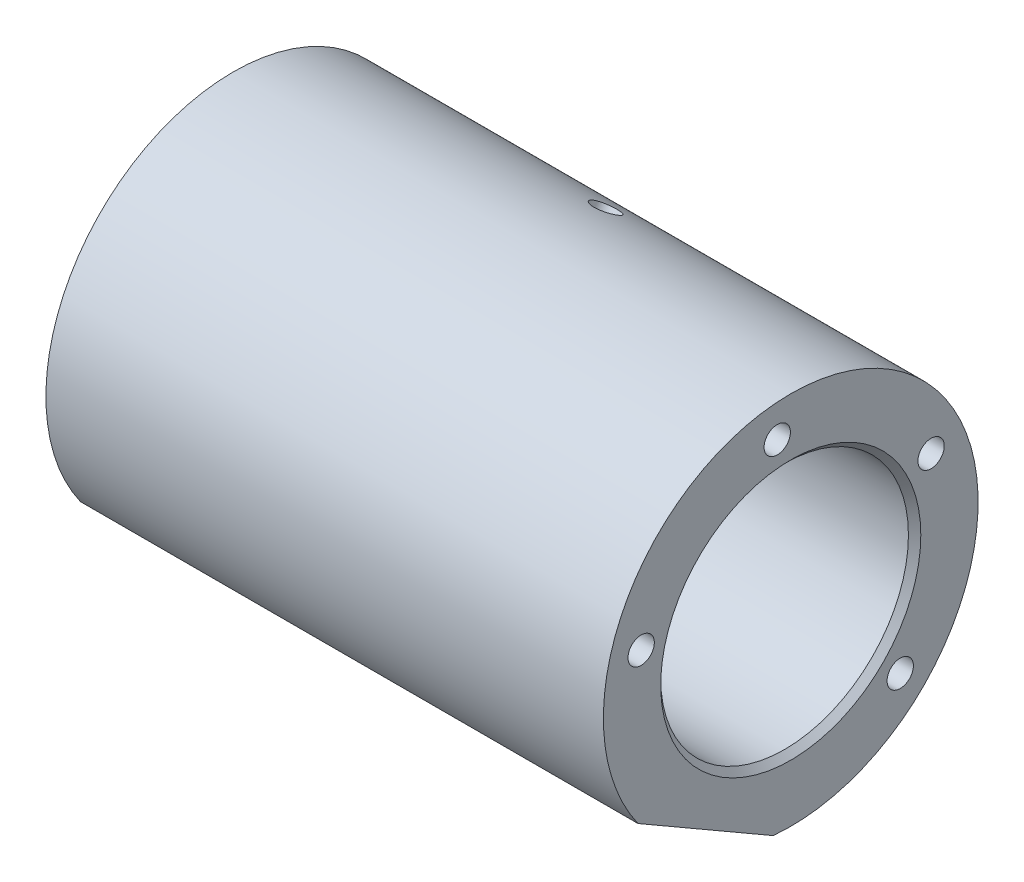
SolidWorks part; units mm, degrees
material "Q345B"
ref_plane "Front Plane" through (0, 0, 0) normal (0, 0, 1) x (1, 0, 0)
ref_plane "Top Plane" through (0, 0, 0) normal (0, 1, 0) x (1, 0, 0)
ref_plane "Right Plane" through (0, 0, 0) normal (1, 0, 0) x (0, 0, -1)
sketch "Sketch1" plane through (0, 0, 0) normal (1, 0, 0) x (0, 0, -1)
  circle A0 centre (0, 0) radius 60.5
  circle A1 centre (0, 0) radius 40
  dimension "D1" = 121
  dimension "D2" = 80
extrude "Boss-Extrude1" add sketch "Sketch1" along normal mid plane 180
sketch "Sketch5" plane through (0, 0, 0) normal (1, 0, 0) x (0, 0, -1)
  line L0 (-49.3274, -35.0293) -> (-5.6726, -60.2335)
  line L1 (-80.485, 0) -> (77.6144, 0) construction
  circle A0 centre (0, 0) radius 60.5 construction
  arc A1 (-49.3274, -35.0293) -> (-5.6726, -60.2335) centre (0, 0) ccw
  dimension "D1" = 30
  dimension "D2" = 55
extrude "Cut-Extrude1" cut sketch "Sketch5" against normal through all both and the other way through all
ref_plane "Plane1" through (0, 0, 0) normal (0, 0.866, -0.5) x (-1, 0, 0)
hole_wizard "M10 Tapped Hole1" positions "Sketch7" profile "Sketch6" tap size "M10" standard "GB"
sketch "Sketch7" plane through (0, 0, 0) normal (0, 0.866, -0.5) x (-1, 0, 0)
  point P0 (0, 0)
sketch "Sketch6" plane through (0, 0, 0) normal (1, 0, 0) x (0, -0.5, -0.866)
  line L0 (0, 0) -> (0, 82.6445)
  line L1 (0, 82.6445) -> (4.25, 82.6445)
  line L2 (4.25, 82.6445) -> (4.25, 0)
  line L5 (4.25, 0) -> (0, 0)
  line L11 (0, -6.35) -> (0, 107.95) construction
  dimension "通孔螺纹孔钻头直径" = 8.5
  dimension "通孔螺纹孔钻头深度" = 82.6445
cosmetic thread "Cosmetic thread1" parameters "D2"=10
hole_wizard "M10 Tapped Hole2" positions "Sketch9" profile "Sketch8" tap size "M10" standard "GB"
sketch "Sketch9" plane through (90, 0, 0) normal (1, 0, 0) x (0, 0, -1)
  line L0 (-22.5, -38.9711) -> (0, 0) construction
  line L3 (-5.6726, -60.2335) -> (-49.3274, -35.0293) construction
  line L4 (0, 0) -> (-6.3063, 72.0811) construction
  line L6 (0, 0) -> (65.5772, 30.5792) construction
  line L7 (0, 0) -> (98.1846, -26.3085) construction
  line L9 (70.0237, -70.0237) -> (0, 0) construction
  circle A0 centre (0, 0) radius 50 construction
  point P0 (-4.3578, 49.8097)
  point P2 (45.3154, 21.1309)
  point P4 (35.3553, -35.3553)
  point P6 (-48.2963, 12.941)
  dimension "D1" = 100
  dimension "D2" = 70
  dimension "D3" = 70
  dimension "D4" = 70
sketch "Sketch8" plane through (90, 49.8097, 4.3578) normal (0, 1, 0) x (0, 0, -1)
  line L0 (0, 0) -> (0, 34.5537)
  line L1 (0, 34.5537) -> (4.25, 32)
  line L2 (4.25, 32) -> (4.25, 0)
  line L5 (4.25, 0) -> (0, 0)
  line L10 (0, 34.5537) -> (-4.25, 32) construction
  line L11 (0, -6.35) -> (0, 107.95) construction
  dimension "螺纹孔钻头直径" = 8.5
  dimension "螺纹孔钻头深度" = 32
  dimension "导头角度" = 118
cosmetic thread "Cosmetic thread2" parameters "D1"=25, "D2"=10
cosmetic thread "Cosmetic thread3" parameters "D1"=25, "D2"=10
cosmetic thread "Cosmetic thread4" parameters "D1"=25, "D2"=10
cosmetic thread "Cosmetic thread5" parameters "D1"=25, "D2"=10
chamfer "Chamfer1" distance 2 angle 45 2 edges at (-90, 0, -40) (90, 0, -40)
